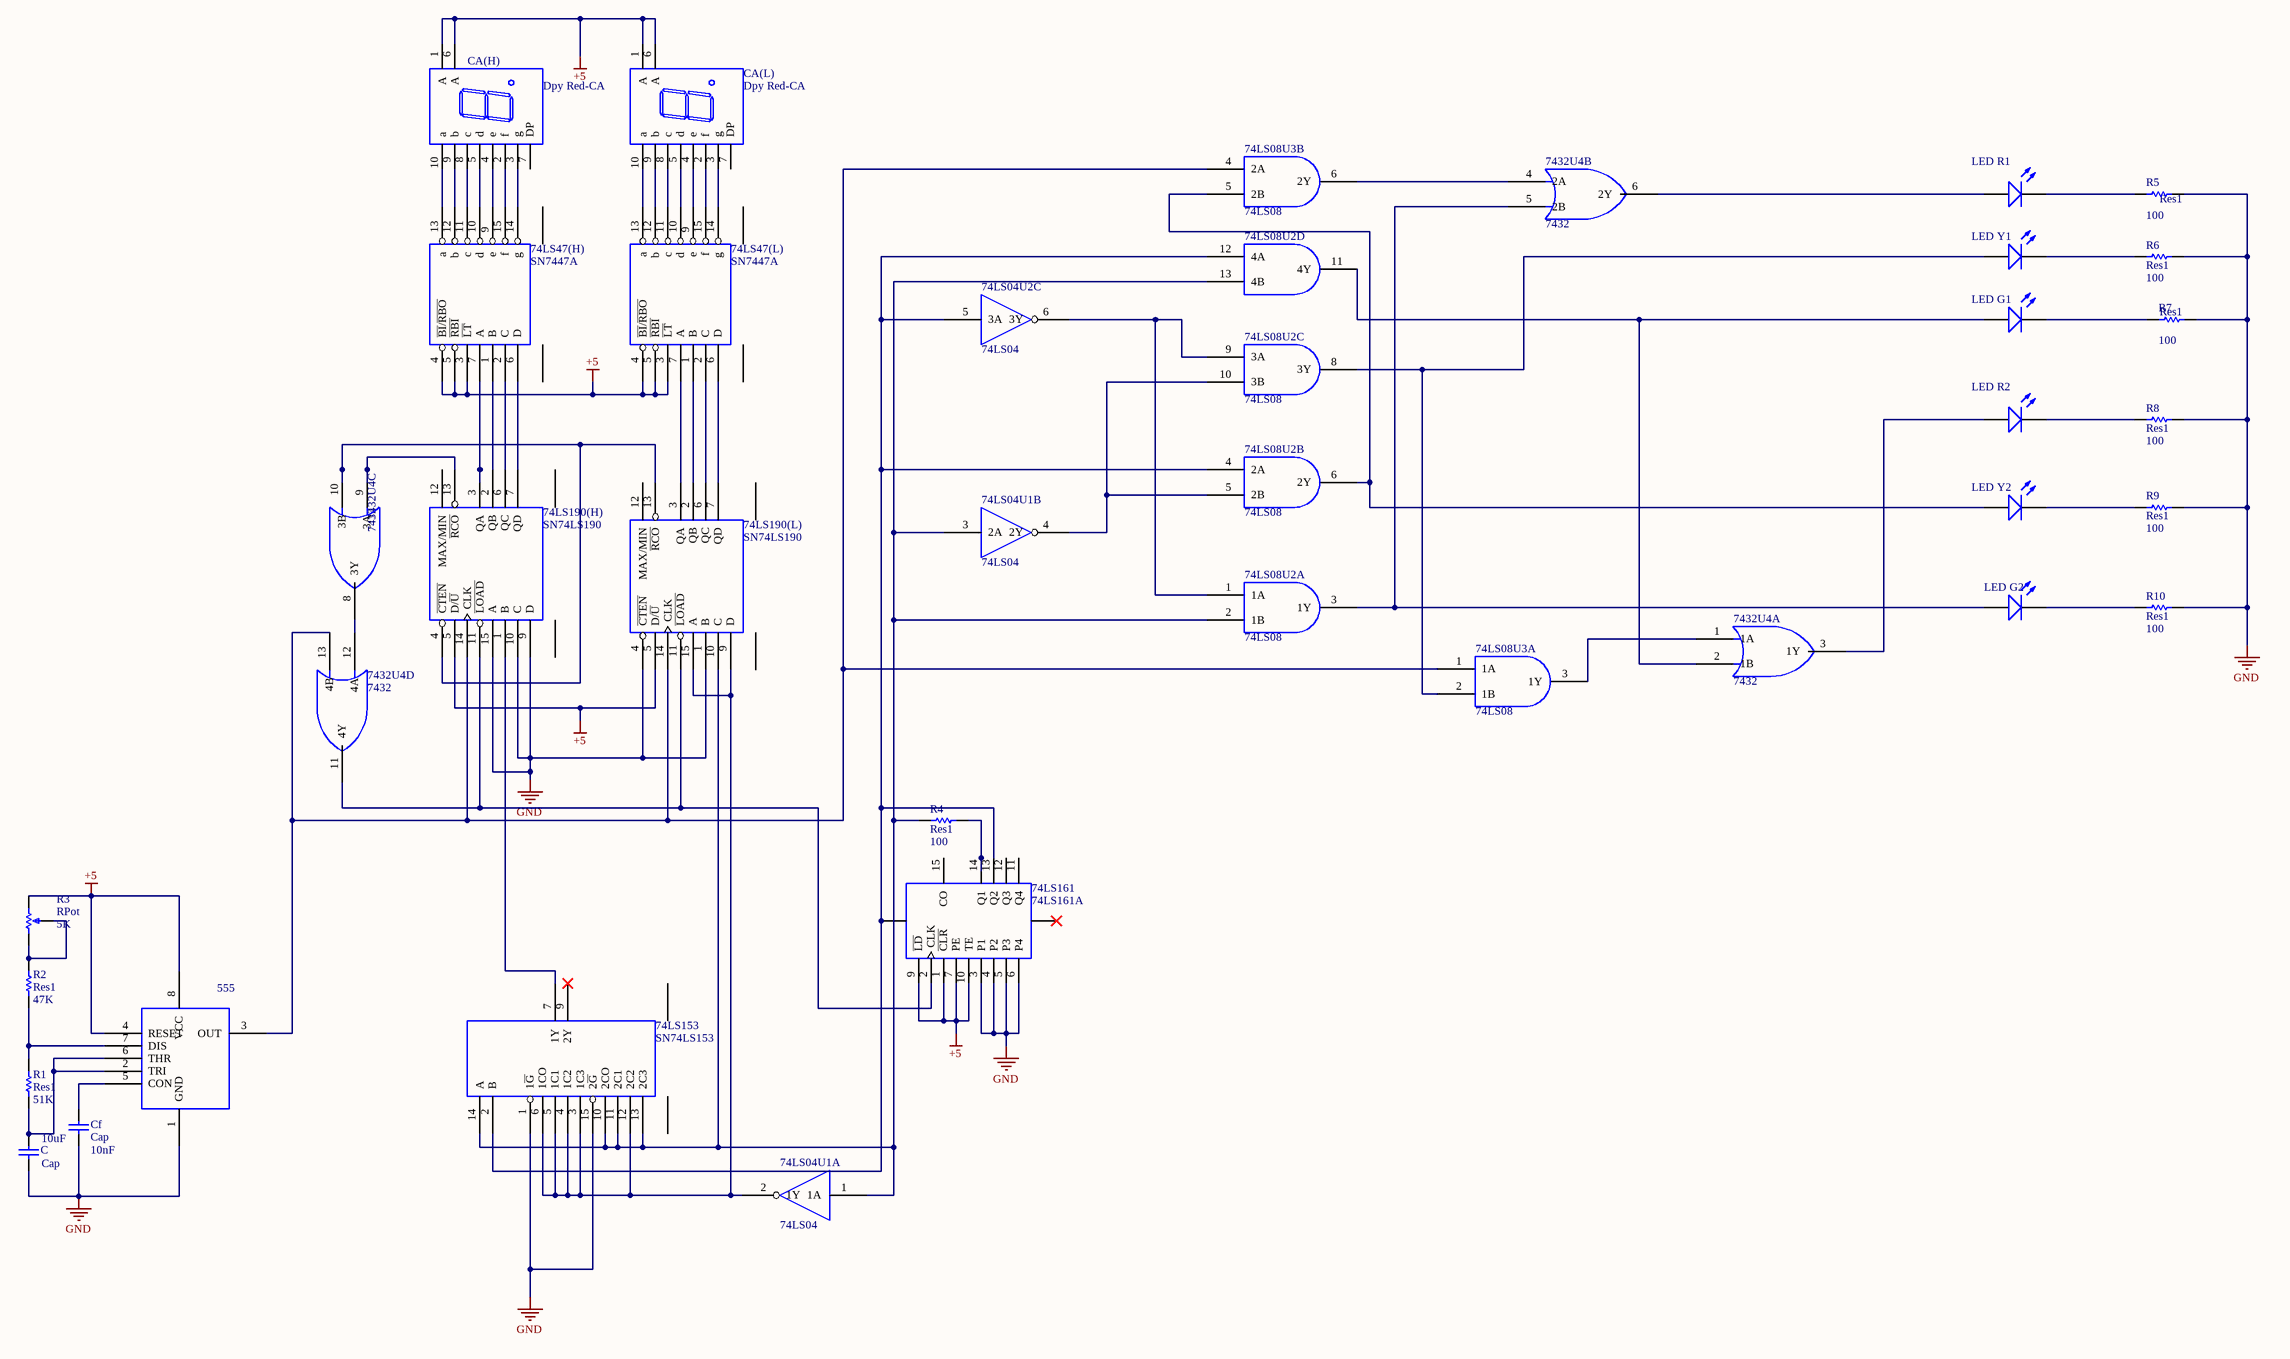
[diagram p0: MISC75419-2.schdoc]
# Altium project MISC75419-3.PrjPcb
1 sheet, 32 parts. Net scope: global (net labels, ports and power ports of the same name join across sheets).
Board file: MISC75419.pcbdoc

## Sheet MISC75419-2.schdoc
size 508 x 381 mm; Name: MISC75419; @Page No: 1; @Page Count: 1; @Schematic Name: MISC75419; @Project Name: MISC75419; @Board Name: MISC75419; @Update Date: 2026-03-27; @Create Time: 22:07:20; @Update Time: 22:07:32; @Create Date: 2026-03-27

### Parts
74LS04U1  74LS04  [DIP14]  (parts A,B of 6)
74LS04U2  74LS04  [DIP14]  (part C of 6)
74LS08U2  74LS08  [DIP14]  (parts A,B,C,D of 4)
74LS08U3  74LS08  [DIP14]  (parts A,B of 4)
74LS47(H)  SN7447A  [DIP16]
74LS47(L)  SN7447A  [DIP16]
74LS153  SN74LS153  [DIP16]
74LS161  74LS161A  [DIP-16]
74LS190(H)  SN74LS190  [DIP-16]
74LS190(L)  SN74LS190  [DIP-16]
555  555  [DIP8]  (value not drawn)
7432U4  7432  [DIP14]  (parts A,B,C,D of 4)
C  Cap  value 10uF  [RAD-0.3]
CA(H)  Dpy Red-CA  [SMG 0.36-1P]
CA(L)  Dpy Red-CA  [SMG 0.36-1P]
Cf  Cap  value 10nF  [RAD-0.3]
LED_G1  LED1_2  [LED-1]  (value not drawn)
LED_G2  LED1_2  [LED-1]  (value not drawn)
LED_R1  LED1  [LED-1]  (value not drawn)
LED_R2  LED1  [LED-1]  (value not drawn)
LED_Y1  LED1_1  [LED-1]  (value not drawn)
LED_Y2  LED1_1  [LED-1]  (value not drawn)
R1  Res1  value 51K  [AXIAL-0.3]
R2  Res1  value 47K  [AXIAL-0.3]
R3  RPot  value 5K  [VR5]
R4  Res1  value 100  [AXIAL-0.3]
R5  Res1  value 100  [AXIAL-0.3]
R6  Res1  value 100  [AXIAL-0.3]
R7  Res1  value 100  [AXIAL-0.3]
R8  Res1  value 100  [AXIAL-0.3]
R9  Res1  value 100  [AXIAL-0.3]
R10  Res1  value 100  [AXIAL-0.3]

### Nets
+5: 74LS47(H).3(~{LT}) 74LS47(H).4(~{BI}/~{RBO}) 74LS47(H).5(~{RBI}) 74LS47(L).3(~{LT}) 74LS47(L).4(~{BI}/~{RBO}) 74LS47(L).5(~{RBI}) 74LS161.1(~{CLR}) 74LS161.7(PE) 74LS161.9(~{LD}) 74LS161.10(TE) 74LS190(H).5(D/~{U}) 74LS190(L).5(D/~{U}) 555.4(RESET) 555.8(VCC) CA(H).1(A) CA(H).6(A) CA(L).1(A) CA(L).6(A) R3.2(BOT)
GND: 74LS153.1(1~{G}) 74LS153.15(2~{G}) 74LS161.3(P1) 74LS161.4(P2) 74LS161.5(P3) 74LS161.6(P4) 74LS190(H).9(D) 74LS190(H).10(C) 74LS190(H).15(A) 74LS190(L).1(B) 74LS190(L).4(~{CTEN}) 555.1(GND) C.1 Cf.1 R5.2 R6.2 R7.2 R8.2 R9.2 R10.2
Net74LS04U1_1: 74LS04U1.1(1A) 74LS04U1.3(2A) 74LS08U2.2(1B) 74LS08U2.13(4B) 74LS153.10(2CO) 74LS153.11(2C1) 74LS153.13(2C3) 74LS153.14(A) 74LS190(L).10(C) R4.1
Net74LS04U1_2: 74LS04U1.2(1Y) 74LS153.3(1C3) 74LS153.4(1C2) 74LS153.5(1C1) 74LS153.6(1CO) 74LS153.12(2C2) 74LS190(L).9(D) 74LS190(L).15(A)
Net74LS04U1_4: 74LS04U1.4(2Y) 74LS08U2.5(2B) 74LS08U2.10(3B)
Net74LS04U2_5: 74LS04U2.5(3A) 74LS08U2.4(2A) 74LS08U2.12(4A) 74LS153.2(B) 74LS161.13(Q2) 74LS161.16(VCC)
Net74LS04U2_6: 74LS04U2.6(3Y) 74LS08U2.1(1A) 74LS08U2.9(3A)
Net74LS08U2_3: 74LS08U2.3(1Y) 7432U4.5(2B) LED_G2.1(A)
Net74LS08U2_6: 74LS08U2.6(2Y) 74LS08U3.5(2B) LED_Y2.1(A)
Net74LS08U2_8: 74LS08U2.8(3Y) 74LS08U3.2(1B) LED_Y1.1(A)
Net74LS08U2_11: 74LS08U2.11(4Y) 7432U4.2(1B) LED_G1.1(A)
Net74LS08U3_1: 74LS08U3.1(1A) 74LS08U3.4(2A) 74LS190(H).14(CLK) 74LS190(L).14(CLK) 555.3(OUT) 7432U4.13(4B)
Net74LS08U3_3: 74LS08U3.3(1Y) 7432U4.1(1A)
Net74LS08U3_6: 74LS08U3.6(2Y) 7432U4.4(2A)
Net74LS47(H)_1: 74LS47(H).1(B) 74LS190(H).2(QB)
Net74LS47(H)_2: 74LS47(H).2(C) 74LS190(H).6(QC)
Net74LS47(H)_6: 74LS47(H).6(D) 74LS190(H).7(QD)
Net74LS47(H)_7: 74LS47(H).7(A) 74LS190(H).3(QA)
Net74LS47(H)_9: 74LS47(H).9(e) CA(H).4(e)
Net74LS47(H)_10: 74LS47(H).10(d) CA(H).5(d)
Net74LS47(H)_11: 74LS47(H).11(c) CA(H).8(c)
Net74LS47(H)_12: 74LS47(H).12(b) CA(H).9(b)
Net74LS47(H)_13: 74LS47(H).13(a) CA(H).10(a)
Net74LS47(H)_14: 74LS47(H).14(g) CA(H).3(g)
Net74LS47(H)_15: 74LS47(H).15(f) CA(H).2(f)
Net74LS47(L)_1: 74LS47(L).1(B) 74LS190(L).2(QB)
Net74LS47(L)_2: 74LS47(L).2(C) 74LS190(L).6(QC)
Net74LS47(L)_6: 74LS47(L).6(D) 74LS190(L).7(QD)
Net74LS47(L)_7: 74LS47(L).7(A) 74LS190(L).3(QA)
Net74LS47(L)_9: 74LS47(L).9(e) CA(L).4(e)
Net74LS47(L)_10: 74LS47(L).10(d) CA(L).5(d)
Net74LS47(L)_11: 74LS47(L).11(c) CA(L).8(c)
Net74LS47(L)_12: 74LS47(L).12(b) CA(L).9(b)
Net74LS47(L)_13: 74LS47(L).13(a) CA(L).10(a)
Net74LS47(L)_14: 74LS47(L).14(g) CA(L).3(g)
Net74LS47(L)_15: 74LS47(L).15(f) CA(L).2(f)
Net74LS153_7: 74LS153.7(1Y) 74LS190(H).1(B)
Net74LS161_2: 74LS161.2(CLK) 74LS190(H).11(~{LOAD}) 74LS190(L).11(~{LOAD}) 7432U4.11(4Y)
Net74LS161_14: 74LS161.14(Q1) R4.2
Net74LS190(H)_4: 74LS190(H).4(~{CTEN}) 74LS190(L).13(~{RCO}) 7432U4.10(3B)
Net74LS190(H)_13: 74LS190(H).13(~{RCO}) 7432U4.9(3A)
Net555_2: 555.2(TRI) 555.6(THR) C.2 R1.1
Net555_5: 555.5(CON) Cf.2
Net555_7: 555.7(DIS) R1.2 R2.1
Net7432U4_3: 7432U4.3(1Y) LED_R2.1(A)
Net7432U4_6: 7432U4.6(2Y) LED_R1.1(A)
Net7432U4_8: 7432U4.8(3Y) 7432U4.12(4A)
NetLED_G1_2: LED_G1.2(K) R7.1
NetLED_G2_2: LED_G2.2(K) R10.1
NetLED_R1_2: LED_R1.2(K) R5.1
NetLED_R2_2: LED_R2.2(K) R8.1
NetLED_Y1_2: LED_Y1.2(K) R6.1
NetLED_Y2_2: LED_Y2.2(K) R9.1
NetR2_2: R2.2 R3.1(TOP) R3.3(TAP)

Not connected (* = marked no-connect by the designer): 74LS47(H) 8(GND) 16(VCC); 74LS47(L) 8(GND) 16(VCC); 74LS153 8(GND) 9(2Y)* 16(VCC); 74LS161 8(GND)* 11(Q4) 12(Q3) 15(CO); 74LS190(H) 8(GND) 12(MAX/MIN) 16(VCC); 74LS190(L) 8(GND) 12(MAX/MIN) 16(VCC); CA(H) 7(DP); CA(L) 7(DP)

### Notes on the sheet
- Title
- Size:
- Date:
- File:
- *
- C
- Number:
- Time:
- Revision:
- Sheet
- of
- NSW

### Library data of the parts
74LS04U1 = 74LS04: Convert to PCB: yes; Device: 74LS04; DesignItemID: 74LS04; LibraryName: shudian; SymbolName: 74LS04; FootprintName: DIP14; AddInBom: yes
74LS04U2 = 74LS04: AddInBom: yes; Device: 74LS04; DesignItemID: 74LS04; LibraryName: shudian; SymbolName: 74LS04; FootprintName: DIP14
74LS08U2 = 74LS08: AddInBom: yes; Device: 74LS08; DesignItemID: 74LS08; LibraryName: shudian; SymbolName: 74LS08; FootprintName: DIP14
74LS08U3 = 74LS08: Convert to PCB: yes; Device: 74LS08; DesignItemID: 74LS08; LibraryName: shudian; SymbolName: 74LS08; FootprintName: DIP14; AddInBom: yes
74LS47(H) = SN7447A: BCD-To-SEVEN-SEGMENT DEC DRV; Origin Footprint: DIP-16; OriginFootprint 2: SO16; SymbolName: SN7446A; AddInBom: yes; Device: SN7447A; DesignItemID: SN7446A; LibraryName: 1.4 - 74 series TTL chips; FootprintName: DIP16
74LS47(L) = SN7447A: BCD-To-SEVEN-SEGMENT DEC DRV; Origin Footprint: SO16; SymbolName: SN7446A; AddInBom: yes; Device: SN7447A; DesignItemID: SN7446A; LibraryName: 1.4 - 74 series TTL chips; FootprintName: DIP16; OriginFootprint 2: SO16
74LS153 = SN74LS153: DUAL 4-1 LINE DATA SELEC/MUX; Origin Footprint: SO16; OriginFootprint 2: DIP-16; AddInBom: yes; Device: SN74LS153; DesignItemID: SN74LS153; LibraryName: 1.4 - 74 series TTL chips; SymbolName: SN74LS153; FootprintName: DIP16
74LS161 = 74LS161A: Synchronous 4-Bit Binary Counter with Direct Clear; AddInBom: yes; Device: 74LS161A; DesignItemID: 74LS161A; LibraryName: 1.4 - 74 series TTL chips; SymbolName: 74LS161A; FootprintName: DIP-16
74LS190(H) 74LS190(L) = SN74LS190: SYN UP/DOWN CNT DOWN/UP MODE CONTTOL; Origin Footprint: SO16; AddInBom: yes; Device: SN74LS190; DesignItemID: SN74LS190; LibraryName: 1.4 - 74 series TTL chips; SymbolName: SN74LS190; FootprintName: DIP-16
555 = 555: AddInBom: yes; Device: 555; DesignItemID: 555; LibraryName: Schlib1; SymbolName: 555; FootprintName: DIP8
7432U4 = 7432: Convert to PCB: yes; Device: 7432; DesignItemID: 7432; LibraryName: shudian; SymbolName: 7432; FootprintName: DIP14; AddInBom: yes
C = Cap_1: Capacitor; AddInBom: yes; Device: Cap_1; Published: 8-Jun-2000; LatestRevisionDate: 17-Jul-2002; LatestRevisionNote: Re-released for DXP Platform.; PackageReference: RAD-0.3; PackageDescription: Radial Cap, Thru-Hole; 2 Leads; 0.3 in Pin Spacing; DesignItemID: Cap; LibraryName: Miscellaneous Devices; SymbolName: Cap; FootprintName: RAD-0.3; Publisher: Altium Limited
CA(H) = Dpy Red-CA: 7.62 mm Black Surface HER 7-Segment Display: CA, RH DP; MinimumIntensity: 360 ucd; Note: IF = 5 mA; Note_1: Pins 1 and 6 are redundant Anodes.; Origin Footprint: A; Convert to PCB: yes; Device: Dpy Red-CA; Published: 8-Jun-2000; LatestRevisionDate: 17-Dec-2003; LatestRevisionNote: Schematic revised, PCB Footprint replaced.; DatasheetVersion: 19-Feb-2002; PackageVersion: 11-Feb-2002; PackageReference: A; PackageDescription: LED, 7-Segment Display, 7.62 mm, RHD; 10 Leads; Row Space 5.08 mm; Pitch 2.54 mm; Colour: High Efficiency Red (HER); ComponentLink1Description: Manufacturer Link; DesignItemID: Dpy Red-CA; LibraryName: Miscellaneous Devices; SymbolName: Dpy Red-CA; AddInBom: yes; Publisher: Altium Limited
CA(L) = Dpy Red-CA_1: 7.62 mm Black Surface HER 7-Segment Display: CA, RH DP; MinimumIntensity: 360 ucd; Note: IF = 5 mA; Note_1: Pins 1 and 6 are redundant Anodes.; Origin Footprint: A; Convert to PCB: yes; Device: Dpy Red-CA_1; Published: 8-Jun-2000; LatestRevisionDate: 17-Dec-2003; LatestRevisionNote: Schematic revised, PCB Footprint replaced.; DatasheetVersion: 19-Feb-2002; PackageVersion: 11-Feb-2002; PackageReference: A; PackageDescription: LED, 7-Segment Display, 7.62 mm, RHD; 10 Leads; Row Space 5.08 mm; Pitch 2.54 mm; Colour: High Efficiency Red (HER); ComponentLink1Description: Manufacturer Link; DesignItemID: Dpy Red-CA; LibraryName: Miscellaneous Devices; SymbolName: Dpy Red-CA; AddInBom: yes; Publisher: Altium Limited
Cf = Cap: Capacitor; AddInBom: yes; Device: Cap; Published: 8-Jun-2000; LatestRevisionDate: 17-Jul-2002; LatestRevisionNote: Re-released for DXP Platform.; PackageReference: RAD-0.3; PackageDescription: Radial Cap, Thru-Hole; 2 Leads; 0.3 in Pin Spacing; DesignItemID: Cap; LibraryName: Miscellaneous Devices; SymbolName: Cap; FootprintName: RAD-0.3; Publisher: Altium Limited
LED_G1 LED_G2 = LED1_2: Typical RED GaAs LED; SymbolName: LED1; AddInBom: yes; Device: LED1_2; Published: 8-Jun-2000; LatestRevisionDate: 08-Jul-2005; LatestRevisionNote: Mech Layer 1 removed.; PackageReference: LED-1; PackageDescription: LED; 2 Leads; DesignItemID: LED1; LibraryName: Miscellaneous Devices; FootprintName: LED-1; Publisher: Altium Limited
LED_R1 LED_R2 = LED1: Typical RED GaAs LED; AddInBom: yes; Device: LED1; Published: 8-Jun-2000; LatestRevisionDate: 08-Jul-2005; LatestRevisionNote: Mech Layer 1 removed.; PackageReference: LED-1; PackageDescription: LED; 2 Leads; DesignItemID: LED1; LibraryName: Miscellaneous Devices; SymbolName: LED1; FootprintName: LED-1; Publisher: Altium Limited
LED_Y1 LED_Y2 = LED1_1: Typical RED GaAs LED; SymbolName: LED1; AddInBom: yes; Device: LED1_1; Published: 8-Jun-2000; LatestRevisionDate: 08-Jul-2005; LatestRevisionNote: Mech Layer 1 removed.; PackageReference: LED-1; PackageDescription: LED; 2 Leads; DesignItemID: LED1; LibraryName: Miscellaneous Devices; FootprintName: LED-1; Publisher: Altium Limited
R1 R2 R4-R10 = Res1: Resistor; AddInBom: yes; Device: Res1; Published: 8-Jun-2000; LatestRevisionDate: 17-Jul-2002; LatestRevisionNote: Re-released for DXP Platform.; PackageReference: AXIAL-0.3; PackageDescription: Axial Device, Thru-Hole; 2 Leads; 0.3 in Pin Spacing; DesignItemID: Res1; LibraryName: Miscellaneous Devices; SymbolName: Res1; FootprintName: AXIAL-0.3; Publisher: Altium Limited
R3 = RPot: Potentiometer; Sim Note: Enter the Resistance value and the set point into parameter fields.; Set Position: 0.5; AddInBom: yes; Device: RPot; Published: 8-Jun-2000; LatestRevisionDate: 17-Jul-2002; LatestRevisionNote: Re-released for DXP Platform.; PackageReference: VR5; PackageDescription: Variable Resistor, Thru-Hole; 3 Leads; DesignItemID: RPot; LibraryName: Miscellaneous Devices; SymbolName: RPot; FootprintName: VR5; Publisher: Altium Limited